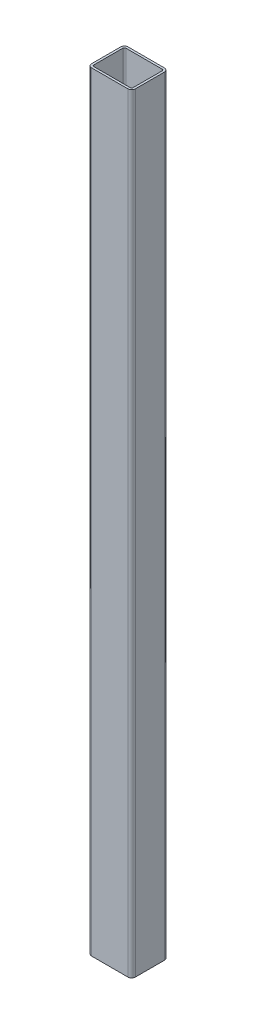
from build123d import *

# Parameters (mm, degrees)
EXTRUDE_THIN1_DEPTH = 1057


with BuildPart() as part:
    # Sketch1 → Extrude-Thin1 (new, symmetric)
    with BuildSketch(Plane(origin=(0, 0, 0), x_dir=(1, 0, 0), z_dir=(0, 1, 0))):
        with BuildLine():
            Line((-50, 50), (50, 50))
            ThreePointArc((50, 50), (57.071067812, 47.071067812), (60, 40))
            Line((60, 40), (60, -40))
            ThreePointArc((60, -40), (57.071067812, -47.071067812), (50, -50))
            Line((50, -50), (-50, -50))
            ThreePointArc((-50, -50), (-57.071067812, -47.071067812), (-60, -40))
            Line((-60, -40), (-60, 40))
            ThreePointArc((-60, 40), (-57.071067812, 47.071067812), (-50, 50))
        make_face()
        with BuildLine():
            Line((-50, 44), (50, 44))
            ThreePointArc((50, 44), (52.828427125, 42.828427125), (54, 40))
            Line((54, 40), (54, -40))
            ThreePointArc((54, -40), (52.828427125, -42.828427125), (50, -44))
            Line((50, -44), (-50, -44))
            ThreePointArc((-50, -44), (-52.828427125, -42.828427125), (-54, -40))
            Line((-54, -40), (-54, 40))
            ThreePointArc((-54, 40), (-52.828427125, 42.828427125), (-50, 44))
        make_face(mode=Mode.SUBTRACT)
    extrude(amount=EXTRUDE_THIN1_DEPTH, both=True)


solid = part.part
